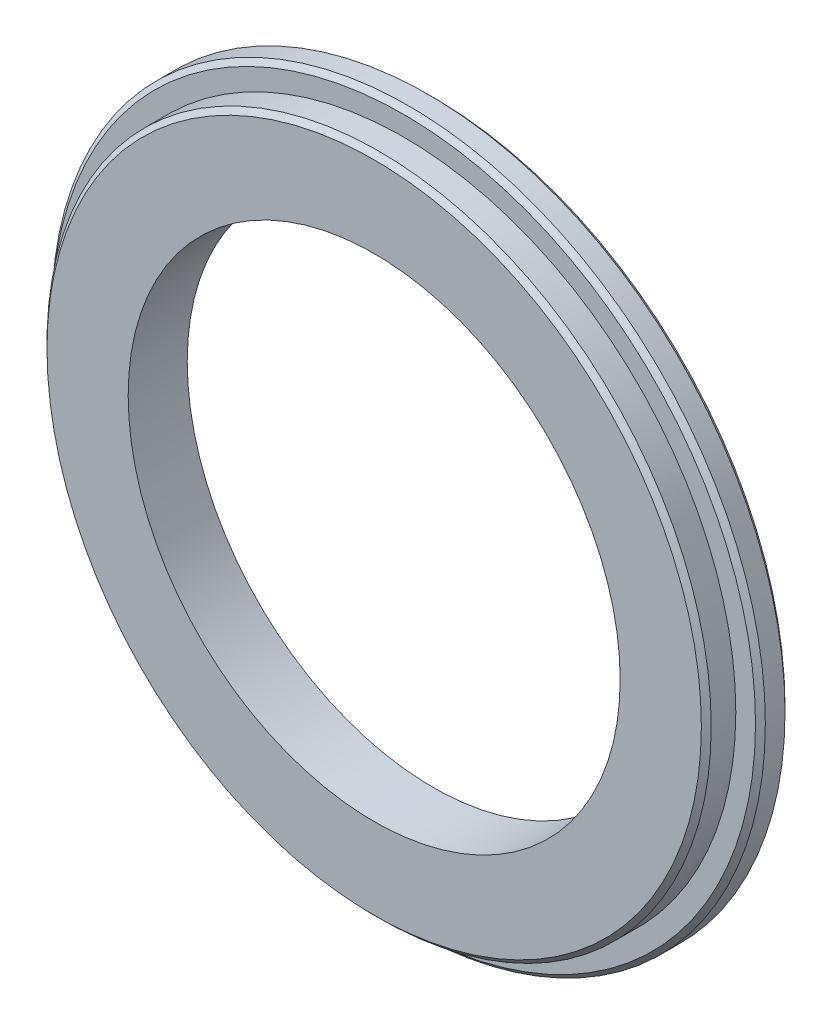
SolidWorks part; units mm, degrees
material "Q235B"
ref_plane "Front Plane" through (0, 0, 0) normal (0, 0, 1) x (1, 0, 0)
ref_plane "Top Plane" through (0, 0, 0) normal (0, 1, 0) x (1, 0, 0)
ref_plane "Right Plane" through (0, 0, 0) normal (1, 0, 0) x (0, 0, -1)
sketch "Sketch1" plane through (0, 0, 0) normal (0, 0, 1) x (1, 0, 0)
  circle A0 centre (0, 0) radius 72.5
  circle A1 centre (0, 0) radius 50
  dimension "D1" = 100
  dimension "D2" = 145
extrude "Boss-Extrude1" add sketch "Sketch1" along normal blind 6
sketch "Sketch2" plane through (0, 0, 6) normal (0, 0, 1) x (1, 0, 0)
  circle A0 centre (0, 0) radius 50
  circle A1 centre (0, 0) radius 67.5
  dimension "D1" = 135
  dimension "D2" = 100
extrude "Boss-Extrude2" add sketch "Sketch2" along normal blind 6
chamfer "Chamfer1" distance 1 distance2 1 3 edges at (72.5, 0, 0) (72.5, 0, 6) (67.5, 0, 12)
sketch "Sketch3" plane through (0, 0, 0) normal (0, 0, -1) x (-1, 0, 0)
  circle A0 centre (-30, 51.9615) radius 3
  circle A4 centre (-60, 0) radius 3
  circle A7 centre (30, 51.9615) radius 3
  circle A8 centre (60, 0) radius 3
  circle A9 centre (30, -51.9615) radius 3
  circle A10 centre (-30, -51.9615) radius 3
  point P17 (65, 0)
  dimension "D3" = 60
  dimension "D4" = 6
extrude "Cut-Extrude1" cut sketch "Sketch3" against normal blind 8
hole_wizard "M8 Tapped Hole1" positions "Sketch4" profile "Sketch5" tap size "M8" standard "GB"
sketch "Sketch4" plane through (0, 0, 0) normal (0, 0, -1) x (-1, 0, 0)
  point P0 (-30, 51.9615)
  point P3 (30, 51.9615)
  point P6 (60, 0)
  point P9 (30, -51.9615)
  point P12 (-30, -51.9615)
  point P15 (-60, 0)
sketch "Sketch5" plane through (30, 51.9615, 0) normal (1, 0, 0) x (0, 1, 0)
  line L0 (0, 0) -> (0, 10.0429)
  line L1 (0, 10.0429) -> (3.4, 8)
  line L2 (3.4, 8) -> (3.4, 0)
  line L5 (3.4, 0) -> (0, 0)
  line L10 (0, 10.0429) -> (-3.4, 8) construction
  line L11 (0, -6.35) -> (0, 107.95) construction
  dimension "螺纹孔钻头直径" = 6.8
  dimension "螺纹孔钻头深度" = 8
  dimension "导头角度" = 118
cosmetic thread "Cosmetic thread1" parameters "D1"=8, "D2"=7.723
cosmetic thread "Cosmetic thread2" parameters "D1"=8, "D2"=7.723
cosmetic thread "Cosmetic thread3" parameters "D1"=8, "D2"=7.723
cosmetic thread "Cosmetic thread4" parameters "D1"=8, "D2"=7.723
cosmetic thread "Cosmetic thread5" parameters "D1"=8, "D2"=7.723
cosmetic thread "Cosmetic thread6" parameters "D1"=8, "D2"=7.723
